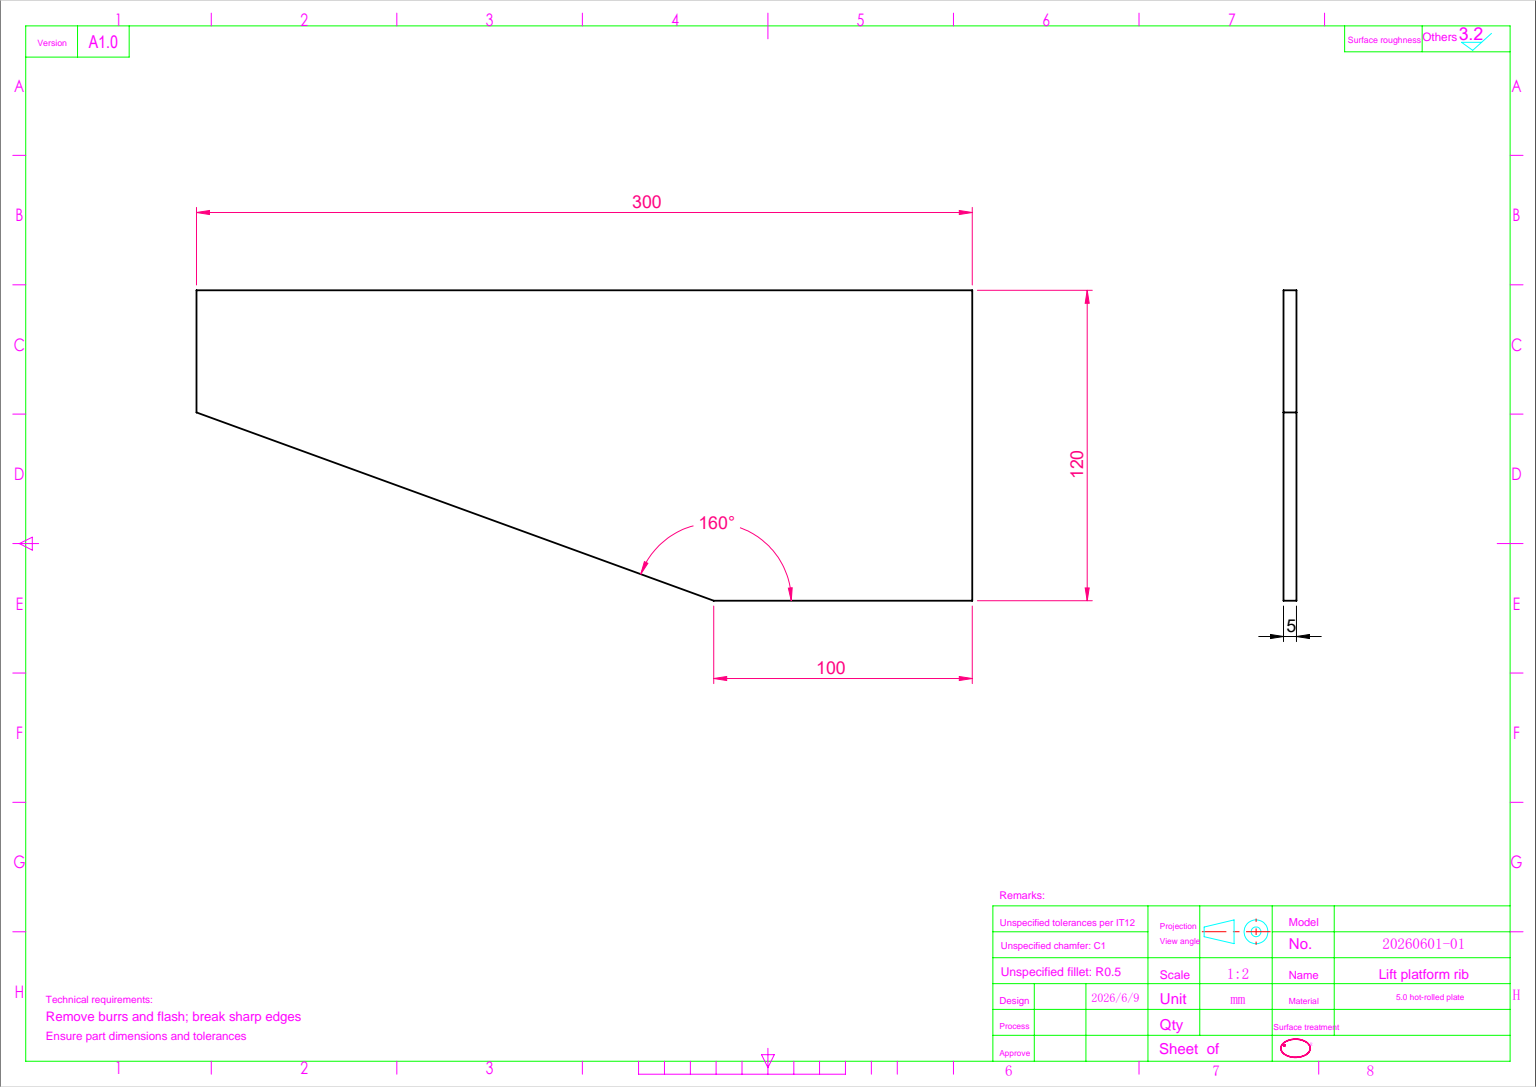
from build123d import *

# Parameters (mm, degrees)
EXTRUDE_1_DEPTH = 5


with BuildPart() as part:
    # 草图1 → 凸台-拉伸1 (new body)
    with BuildSketch(Plane.XY):
        Polygon((0, 0), (300, 0), (300, -120), (200, -120), (0, -47.205953147), align=None)
    extrude(amount=EXTRUDE_1_DEPTH)


solid = part.part
